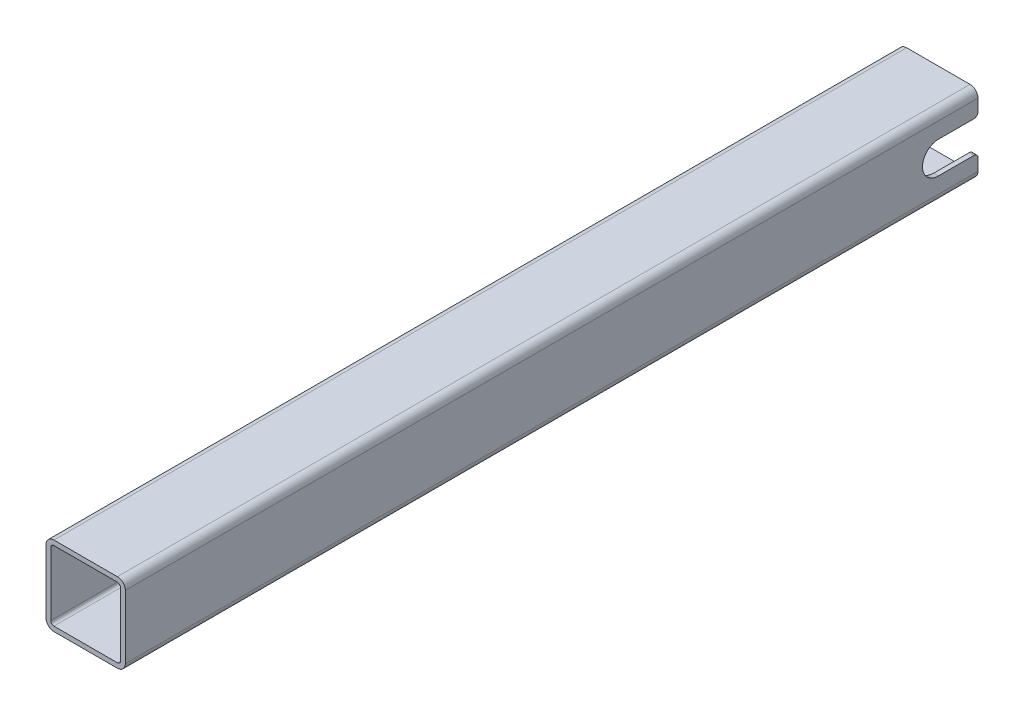
from build123d import *

# Parameters (mm, degrees)
EXTRUDE_1_DEPTH     = 2150
CUT_EXTRUDE_2_DEPTH = 12
FILLET_1_R          = 10


with BuildPart() as part:
    # 草图1 → 凸台-拉伸1 (new body)
    with BuildSketch(Plane.XY):
        with BuildLine():
            Line((-80, 100), (80, 100))
            ThreePointArc((80, 100), (94.142135624, 94.142135624), (100, 80))
            Line((100, 80), (100, -80))
            ThreePointArc((100, -80), (94.142135624, -94.142135624), (80, -100))
            Line((80, -100), (-80, -100))
            ThreePointArc((-80, -100), (-94.142135624, -94.142135624), (-100, -80))
            Line((-100, -80), (-100, 80))
            ThreePointArc((-100, 80), (-94.142135624, 94.142135624), (-80, 100))
        make_face()
        with BuildLine():
            Line((-80, 88), (80, 88))
            ThreePointArc((80, 88), (85.656854249, 85.656854249), (88, 80))
            Line((88, 80), (88, -80))
            ThreePointArc((88, -80), (85.656854249, -85.656854249), (80, -88))
            Line((80, -88), (-80, -88))
            ThreePointArc((-80, -88), (-85.656854249, -85.656854249), (-88, -80))
            Line((-88, -80), (-88, 80))
            ThreePointArc((-88, 80), (-85.656854249, 85.656854249), (-80, 88))
        make_face(mode=Mode.SUBTRACT)
    extrude(amount=EXTRUDE_1_DEPTH)

    # 草图3 → 切除-拉伸2 (cut)
    with BuildSketch(Plane(origin=(100, 0, 0), x_dir=(0, 0, -1), z_dir=(1, 0, 0))):
        with BuildLine():
            Line((-100, 40), (100, 40))
            ThreePointArc((100, 40), (140, 0), (100, -40))
            Line((100, -40), (-100, -40))
            ThreePointArc((-100, -40), (-140, 0), (-100, 40))
        make_face()
    extrude(amount=-CUT_EXTRUDE_2_DEPTH, mode=Mode.SUBTRACT)

    # 圆角1
    fillet_1_edges = [part.edges().sort_by_distance(p)[0] for p in [
        (94, -40, 0),
        (94, 40, 0),
    ]]
    fillet(fillet_1_edges, radius=FILLET_1_R)


solid = part.part
